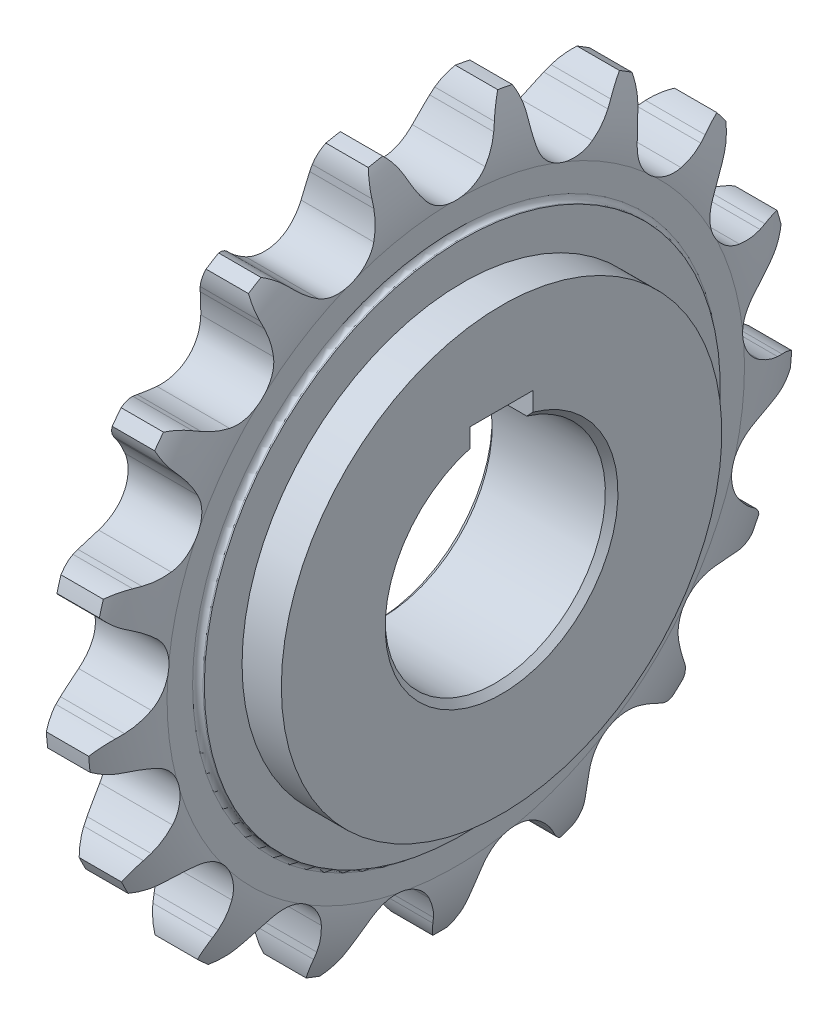
from build123d import *

# Parameters (mm, degrees)
CUT_EXTRUDE_1_DEPTH      = 6.879956443
PATTERN_CIRCULAR_1_COUNT = 17
SKETCH_4_W               = 10
SKETCH_4_H               = 4.029490121
CUT_EXTRUDE_2_DEPTH      = 81.282723363
CHAMFER_1_SIZE           = 1
SKETCH_5_R               = 35
EXTRUDE_1_DEPTH          = 6.24
CHAMFER_4_SIZE           = 1


with BuildPart() as part:
    # 草图1 → 旋转1 (revolve)
    with BuildSketch(Plane.XY, mode=Mode.PRIVATE) as revolve_1_sk:
        with BuildLine():
            Line((-6.879956443, 17.5), (-6.879956443, 41))
            Line((-6.879956443, 41), (-6.672975154, 41))
            ThreePointArc((-6.672975154, 41), (-6.087543663, 41.242493663), (-5.84505, 41.827925154))
            Line((-5.84505, 41.827925154), (-5.84505, 45.88187072))
            ThreePointArc((-5.84505, 45.88187072), (-5.311822172, 51.113495659), (-3.36855, 56))
            Line((-3.36855, 56), (3.36855, 56))
            ThreePointArc((3.36855, 56), (5.311822172, 51.113495659), (5.84505, 45.88187072))
            Line((5.84505, 45.88187072), (5.84505, 41.827925154))
            ThreePointArc((5.84505, 41.827925154), (6.087543663, 41.242493663), (6.672975154, 41))
            Line((6.672975154, 41), (6.879956443, 41))
            Line((6.879956443, 41), (6.879956443, 17.5))
            Line((6.879956443, 17.5), (-6.879956443, 17.5))
        make_face()
    revolve(revolve_1_sk.sketch.rotate(Axis((-9.525, 0, 0), (1, 0, 0)), 90), axis=Axis((-9.525, 0, 0), (1, 0, 0)))

    # 草图2 → 切除-拉伸1 (cut, symmetric)
    with BuildSketch(Plane(origin=(0, 0, 0), x_dir=(0, 0, -1), z_dir=(1, 0, 0))):
        with BuildLine():
            Line((6.783086347, 51.485885439), (7.237937548, 52.516025204))
            ThreePointArc((7.237937548, 52.516025204), (8.056978257, 53.97414887), (9.139183777, 55.249211034))
            ThreePointArc((9.139183777, 55.249211034), (0, 56), (-9.139183777, 55.249211034))
            ThreePointArc((-9.139183777, 55.249211034), (-8.056978257, 53.97414887), (-7.237937548, 52.516025204))
            Line((-7.237937548, 52.516025204), (-6.783086347, 51.485885439))
            ThreePointArc((-6.783086347, 51.485885439), (-5.861506363, 49.715546761), (-4.720935064, 48.077711051))
            ThreePointArc((-4.720935064, 48.077711051), (0, 45.80209572), (4.720935064, 48.077711051))
            ThreePointArc((4.720935064, 48.077711051), (5.861506363, 49.715546761), (6.783086347, 51.485885439))
        make_face()
    cut_extrude_1 = extrude(amount=CUT_EXTRUDE_1_DEPTH, both=True, mode=Mode.SUBTRACT)

    # 阵列(圆周)1: 切除-拉伸1 ×17 about axis
    pattern_circular_1_axis = Axis((0, 0, 0), (1, 0, 0))
    for i in range(1, PATTERN_CIRCULAR_1_COUNT):
        add(cut_extrude_1.rotate(pattern_circular_1_axis, i * 360 / PATTERN_CIRCULAR_1_COUNT), mode=Mode.SUBTRACT)

    # 草图4 → 切除-拉伸2 (cut, through all)
    with BuildSketch(Plane.ZY.offset(6.879956443)):
        with Locations((0, 18.785254892)):
            Rectangle(SKETCH_4_W, SKETCH_4_H)
    extrude(amount=-CUT_EXTRUDE_2_DEPTH, mode=Mode.SUBTRACT)

    # 倒角1
    chamfer_1_edges = [part.edges().sort_by_distance(p)[0] for p in [
        (-6.879956443, -17.5, 0),
    ]]
    chamfer(chamfer_1_edges, length=CHAMFER_1_SIZE)

    # 草图5 → 凸台-拉伸1 (add)
    with BuildSketch(Plane(origin=(6.879956443, 0, 0), x_dir=(0, 0, -1), z_dir=(1, 0, 0))):
        with Locations(Location((0, 0, 0), (0, 0, 180))):
            Circle(SKETCH_5_R)
        with BuildLine():
            Line((-5, 20.799999952), (5, 20.799999952))
            Line((5, 20.799999952), (5, 16.770509831))
            ThreePointArc((5, 16.770509831), (0, -17.5), (-5, 16.770509831))
            Line((-5, 16.770509831), (-5, 20.799999952))
        make_face(mode=Mode.SUBTRACT)
    extrude(amount=EXTRUDE_1_DEPTH)

    # 倒角4
    chamfer_4_edges = [part.edges().sort_by_distance(p)[0] for p in [
        (13.119956443, -17.5, 0),
    ]]
    chamfer(chamfer_4_edges, length=CHAMFER_4_SIZE)


solid = part.part
